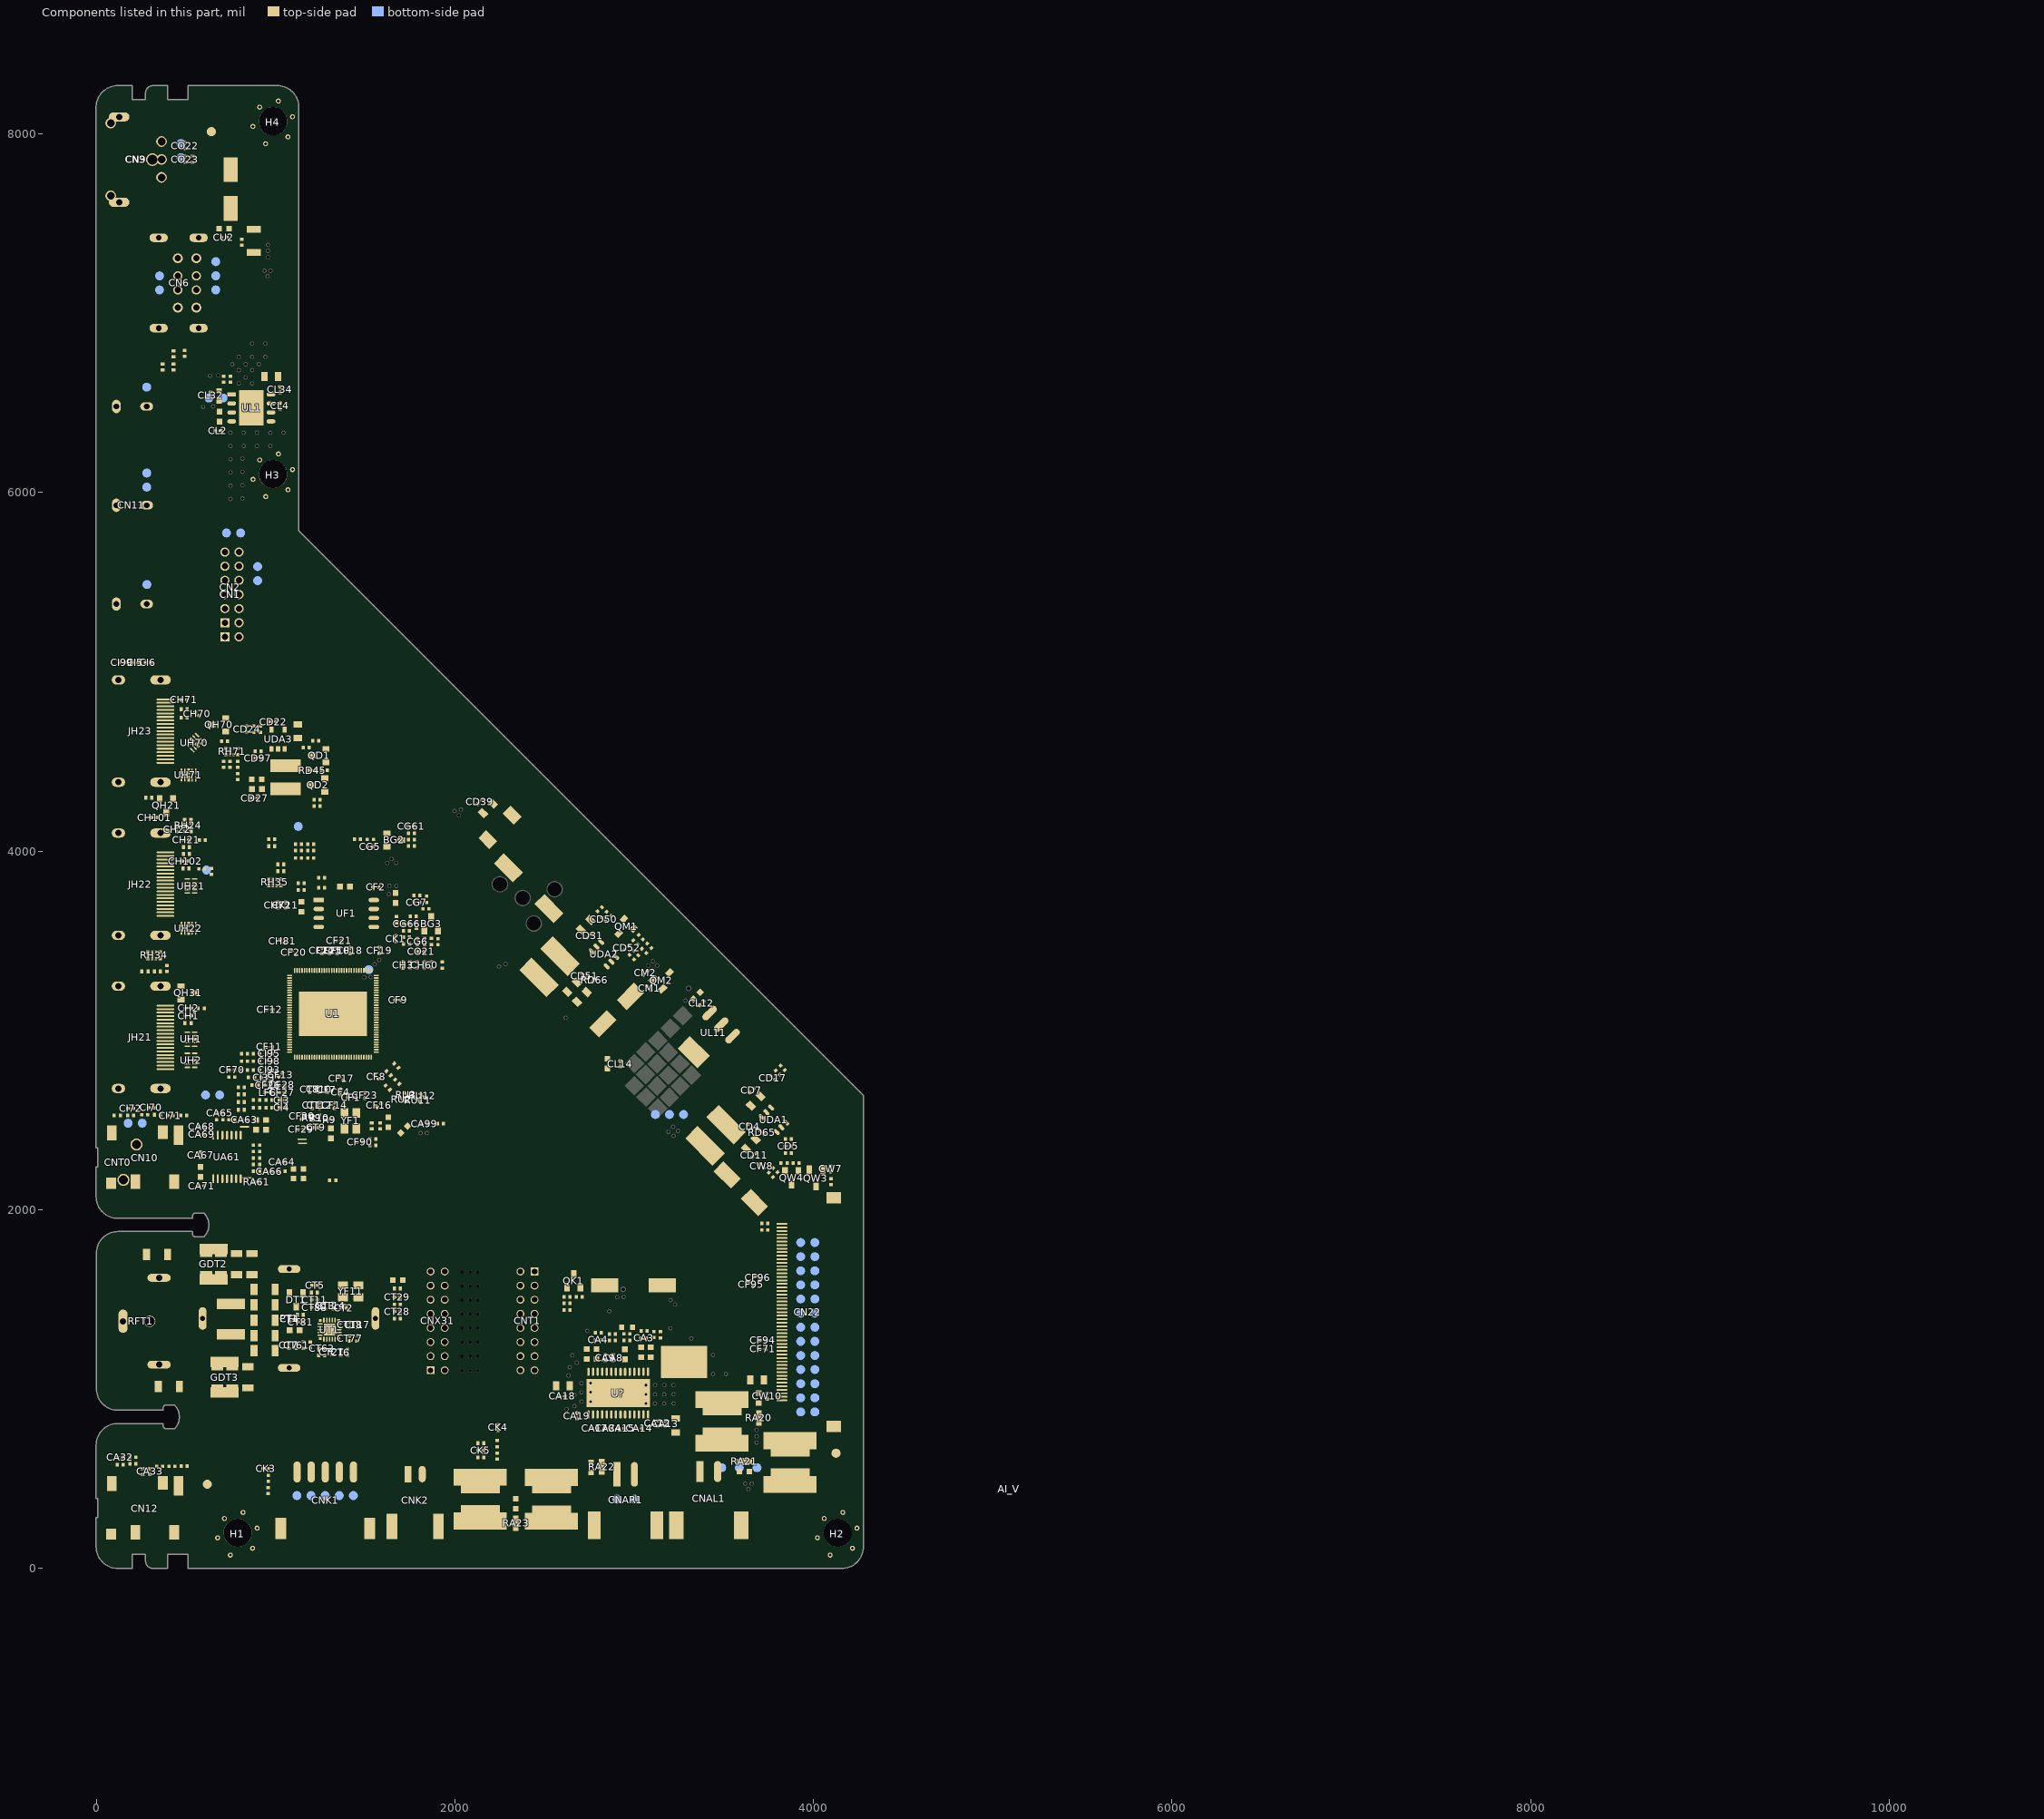
[diagram p0: the components of this part, seen from the top]
# Altium PCB MISC105950.PcbDoc (part 15 of 15)
Units mil, origin at the board's own origin, x right, y up, seen from the top; angles counter-clockwise.
Board outline 4280.62 x 8272.76 mil, 2 copper layers (TopLayer, BottomLayer), stack 61.855 mil thick; 541 components, 268 nets, 2324 pads, 1157 vias.

## Silkscreen, mask and mechanical layers (free items; w line width, h text height)
TopOverlay:
  drawing of 398 lines, arcs and shapes, not listed
  text "Solder Mask:" at 7538.71,8371.14 h60
  text "IPC SM-840" at 7951.21,8370.14 h60
  text "Silkscreen Color:" at 8717.21,8370.14 h60
  text "White" at 9196.21,8370.14 h60
  text "Units:" at 8717.21,8271.14 h60
  text "PTH Copper Thickness:" at 7538.71,8270.14 h60
  text "mm" at 8915.21,8269.64 h60
  text ">20um" at 8212.21,8269.14 h60
  text "4.2 --- 4.6" at 8717.87,8171.67 h60
  text "Dielectric Constant Er@1GHz To 1MHz:" at 7538.37,8171.17 h60
  text "Panel Size:" at 7532,8075.5 h60
  text "2L,2,63.26×214.50mm,FR4(TG130-CTI175),1OZ,Green,OSP,1.6mm" at 8184.37,8062.17 h60
  text "XXXXXXXXXX:" at 7830,8061.5 h60
  text "2L,2,51.80×25.20mm,FR4(TG130-CTI175),1OZ,Green,OSP,1.6mm" at 8184.87,7981.67 h60
  text "XX.XXXX:" at 7858,7975.5 h60
  text "Silkscreen on PTH:" at 7537.21,7871.14 h60
  text "Primary Side Retained;" at 8055.21,7870.14 h60
  text "Secondary Side  Removed for Soldering" at 8717.21,7868.64 h60
  text "Special Requirements" at 7536.19,7780.46 h60
  text "If engineering questions are not answered within 2 hours, call: PHONE_A" at 9422.87,7773.17 h60
  text "1. Lead-free hot air leveling (HAL_LF, Lead Free Hot Air Leveling)" at 8127.09,7676.87 h60
  text "2. Organic solderability preservative (OSP, Organic Solderability Preservatives)" at 8127.09,7592.87 h60
  text "3. Electroless nickel/immersion gold (ENIG, Electroless Nickel/Immersion Gold)" at 8125.59,7501.37 h60
  text "Plated Technics" at 7611.21,7466.64 h60
  text "4. Electroless nickel/immersion gold + gold finger (ENIG_G/F, Electroless Nickel/Immersion Gold + Gold Finger)" at 8127.09,7420.87 h60
  text "5. Gold plated (Gold_plated, Gold-plated)" at 8128.09,7340.37 h60
  text "6. Gold plated + gold finger (Gold_Plated_G/F, Gold-plated + Gold Finger)" at 8128.59,7262.37 h60
  text "Impedance Control" at 7540.94,7033.78 h60
  text "Target Impedance" at 8337.77,7033.88 h60
  text "Width & Clearance" at 9083.6,7033.65 h60
  text "Layer(s)" at 9851.91,7033.96 h60
  text "75 +/- 10% Ohm" at 8350.47,6927.68 h60
  text "G/12/15.8/12/G mil" at 9031.52,6927 h60
  text "layer 1" at 9842.41,6927.12 h60
  text "Single End Impedance" at 7540.94,6886.96 h60
  text "[ Zo ]" at 7764.44,6749.71 h60
  text "G/5/7/5/7/5/G mil" at 9041.52,6536 h60
  text "100 +/- 10% Ohm" at 8337.47,6534.99 h60
  text "layer 1" at 9853.4,6533.21 h60
  text "Differential Impedance" at 7540.8,6485.38 h60
  text "[ Zo ]" at 7763.93,6362.05 h60
  text "( G: Ground )" at 7674.01,6254.55 h60
  text "90 +/- 10% Ohm" at 8363.52,6237 h60
  text "layer 1&2" at 9849.4,6236.21 h60
  text "G/5/11/5/11/5/G mil" at 9041.52,6233.5 h60
  text "Common Mode Impedance" at 7520.58,6032.87 h60
  text "[ Zc ]" at 7768.58,5951.87 h60
  text "MAIN POWER" at 705,5810 h60
  text "INVERTER" at 745,5765 h60
  text "Refer to Gerber documents GTP&GBP for Stencil aperture design" at 8435.63,5687.68 h60
  text "Stencil" at 7534.87,5590.67 h60
  text "New (CN10, CNT0 compatible; note when opening the stencil)" at 8433.53,5493.12 h60
  text "Testing jig" at 7532.96,5395.02 h60
  text "New" at 8435.63,5385.92 h60
  text "Wave-soldering jig" at 7535.17,5296.78 h60
  text "New (when CNX31, CNT1 pass wave soldering, a wave-soldering fixture is required)" at 8425,5297 h60
  text "Solder paste" at 8433.15,5195 h60
  text "Production process" at 7533.65,5193.5 h60
  text "[Process and notes]" at 7713.87,5108.67 h60
  text "SMD parts 3.5mm from PCB edge; production must control specially" at 8432.87,5109.17 h60
  text "Special requirements" at 7534.65,4995.5 h60
  text "SMD parts higher than 2mm on the wave-soldering side" at 7534.37,4894.17 h60
  text "Package attention" at 7534.03,4797.95 h60
  text "[Easily damaged parts]" at 7775.37,4713.17 h60
  text "New footprint matching" at 7534.03,4597.95 h60
  text "RFT1, PT1 are temporary footprints" at 8431.52,4543 h60
  text "[New component footprint]" at 7761.37,4514.17 h60
  text "(Automated Testing Support)" at 7852.37,4399.67 h45
  text "Automated test support" at 7533.87,4396.17 h60
  text "Yes" at 8432.37,4340.17 h60
  text "[Reserved suction cup and press bar positions]" at 7694.37,4311.67 h60
  text "Layer Stack Up Detail for" at 7674.97,3952.14 h100
  text ".Pcb_File_Name_No_Path" at 8735.79,3952.14 h100
  text "Layer" at 7839.33,3804.41 h50
  text "Gerber" at 8211.04,3804.41 h50
  text "Layer" at 8522.19,3804.41 h50
  text "Layer" at 9158.43,3804.41 h50
  text "Copper" at 9947.33,3804.41 h50
  text "Dielectric" at 10259.11,3804.41 h50
  text "Stack up" at 9158.43,3753.53 h50
  text "Height" at 10259.11,3753.53 h50
  text "Name" at 7839.33,3752.03 h50
  text "Document" at 8211.04,3752.03 h50
  text "Ordor" at 8522.19,3752.03 h50
  text "Thickness" at 9947.33,3752.03 h50
  text "TopOverlay" at 7839.03,3519.18 h60
  text ".GTO" at 8248.6,3516.62 h60
  text "0.4mil" at 10256.43,3431.59 h60
  text "1" at 8575.39,3328.44 h60
  text "1.4mil" at 9960.39,3328.38 h60
  text "2" at 8575.45,3115.4 h60
  text "1.4mil" at 9958.68,3114.39 h60
  text "0.4mil" at 10259.1,3019.71 h60
  text "LVDS" at 4195.3,2126.1 h60 r90
  text "ALL SMT" at 1966.7,45.6 h180
  text "SPEAKER _L" at 3275.6,45.2 h60
  text "SPEAKER _R" at 2788.3,39.2 h60
  text "IR&KEY" at 1185.1,35 h60
  text "KEY" at 1724.1,29.1 h60
BottomOverlay:
  drawing of 184 lines, arcs and shapes, not listed
  text "COAX OUT/OPTICAL OUT" at 200.6,7422 h60 r270
  text "USB IN" at 101.9,7093.1 h60 r270
  text "AV IN/YPBPR AUDIO IN" at 162.2,5936.8 h60 r270
  text "BL_ON" at 652.8,5655.1 h50
  text "ADJ/PWM" at 488.3,5652.9 h50
  text "PW_ON" at 656.91,5570.73 h50
  text "GND" at 474.91,5568.43 h50
  text "NC" at 470.9,5493.5 h50
  text "ADIM" at 641.9,5492.9 h50
  text "GND" at 503,5414.9 h50
  text "GND" at 659,5415.4 h50
  text "12V/15V" at 671.5,5338.2 h50
  text "GND" at 487.9,5337.3 h50
  text "12V/15V" at 485.3,5255 h50
  text "12V/15V" at 670.1,5252.4 h50
  text "12V/15V" at 630.4,5172.8 h50
  text "GND" at 448.4,5170.5 h50
  text "HDMI3 IN" at 36.6,4524.9 h60 r270
  text "HDMI2 IN" at 35,3742.6 h60 r270
  text "S.P" at 25.8,3567.3 h90 r270
  text ".GBO" at 8249.22,2924.1 h60
  text "BottomOverlay" at 7827.55,2923.11 h60
  text "HDMI1(ARC) IN" at 38.1,2781.7 h60 r270
  text "YPBPR IN" at 536.21,2178.28 h60
  text "RF IN" at 39.48,1316.39 h60 r270
  text "LOUT-" at 3385.9,631.3 h50 r270
  text "LOUT+" at 3322.7,625 h50 r270
  text "ROUT-" at 2985.66,599.28 h50 r270
  text "ROUT+" at 2890.7,588.7 h50 r270
  text "GND" at 1881,545 h50
  text "KEY" at 1764.7,542 h50
  text "IR" at 1164.6,229.7 h50 r270
  text "3.3V" at 1114.5,215 h50 r270
  text "LED" at 1261.1,214.3 h50 r270
  text "KEY" at 1309,214.3 h50 r270
  text "GND" at 1209.5,209.9 h50 r270
  text "EARPHONE OUT" at 453.4,182.9 h60
  text "LINE OUT" at 366.7,102.7 h60
TopPaste:
  rectangle: 7673.59,3594.48 7803.79,3673.22
  rectangle: 198.7,7809.2 281.5,7907.3
  region: 171,2253.56 123,2253.56 108.5,2239.06 108.5,2211.56 132,2188.06 159.06,2188.06 185,2214 185,2239.56
  lines w5: 8224.49,3594.48 8224.49,3673.22 ; 7673.59,3594.48 7673.59,3673.22 8405.62,3673.22 8405.62,3594.48 7673.59,3594.48
  text "TopPaste" at 7839.03,3615.71 h60
  text ".GTP" at 8248.6,3613.58 h60
BottomPaste:
  rectangle: 7673.59,2806.92 7803.79,2885.66
  lines w5: 8224.49,2806.92 8224.49,2885.66 ; 7673.59,2806.92 7673.59,2885.66 8405.62,2885.66 8405.62,2806.92 7673.59,2806.92
  text "BottomPaste" at 7826.39,2829.9 h60
  text ".GBP" at 8249.49,2824.78 h60
TopSolder:
  rectangle: 7673.59,3404.53 7803.79,3483.27
  lines w5: 8224.49,3404.53 8224.49,3483.27 ; 7673.59,3404.53 7673.59,3483.27 8405.62,3483.27 8405.62,3404.53 7673.59,3404.53
  text "TopSolder" at 7839.53,3424.63 h60
  text ".GTS" at 8248.6,3422.98 h60
BottomSolder:
  rectangle: 7673.59,2994.72 7803.79,3073.46
  region: 1968.4,1049.81 1968.4,971.47 1939.32,923 1859.68,923 1830.6,971.47 1830.6,1049.81
  region: 2469.66,1049.75 2469.66,971.41 2422.41,892.67 2379.11,892.67 2331.86,971.41 2331.86,1049.75
  lines w5: 8224.49,2994.72 8224.49,3073.46 ; 7673.59,2994.72 7673.59,3073.46 8405.62,3073.46 8405.62,2994.72 7673.59,2994.72
  lines w27.56: 210.15,2938.08 338.78,3066.7 ; 210.15,3021.59 255.26,3066.7 ; 210.15,3792.41 338.78,3921.03 ; 210.15,3875.92 255.26,3921.03 ; 210.15,4646.74 338.78,4775.36 ; 210.15,4730.25 255.26,4775.36 ; 210.22,2854.63 421.97,3066.38 ; 210.22,3708.96 421.97,3920.71 ; 210.22,4563.29 421.97,4775.04 ; 293.81,2854.7 422.65,2983.54 ; 293.81,3709.03 422.65,3837.87 ; 293.81,4563.36 422.65,4692.2 ; 377.33,2854.7 422.65,2900.03 ; 377.33,3709.03 422.65,3754.36 ; 377.33,4563.36 422.65,4608.69
  text "BottomSolder" at 7826.39,3016.31 h60
  text ".GBS" at 8248.57,3015.42 h60
3D和装配:
  lines w5: 50.61,2695.01 582.1,2695.01 582.1,3226.51 50.61,3226.51 50.61,2695.01 ; 50.61,3549.34 582.1,3549.34 582.1,4080.84 50.61,4080.84 50.61,3549.34 ; 50.61,4403.67 582.1,4403.67 582.1,4935.17 50.61,4935.17 50.61,4403.67
  text "2L,2,63.26×214.50mm,FR4(TG130-CTI175),1OZ,Green,OSP,1.6mm,4,64,81.3%,1624,0.4mm" at 8184.37,8062.17 h60
  text "2L,2,51.80×25.20mm,FR4(TG130-CTI175),1OZ,Green,OSP,1.6mm,4,64,81.3%,1624,0.4mm" at 8184.87,7981.67 h60
自动测试:
  circle w6: c3435.52,1472.17 r196.85
  circle w6: c595.02,6014.17 r196.85
  circle w6: c596.15,6014.17 r236.22
  circle w6: c1555.85,4758.34 r196.85
  circle w6: c1556.98,4758.34 r236.22
  circle w6: c778.52,3386.67 r196.85
  circle w6: c779.65,3386.67 r236.22
  circle w6: c2342.52,2795.67 r196.85
  circle w6: c2343.65,2795.67 r236.22
  circle w6: c3073.65,2057.17 r236.22
  circle w6: c3072.52,2057.17 r196.85
  circle w6: c899.15,7040 r196.85
顶层限制:
  drawing of 4128 lines, arcs and shapes, not listed
  text "28.6" at 562.99,8601.63 h98.43
  text "25" at 492.13,8365.41 h98.43
  text "1.5" at -505.8,7497.38 h98.43
  text "25" at 411.2,6220.76 h98.43
  text "1.5" at -509.8,4972.38 h98.43
  text "210" at -3064.65,4084.65 h98.43
  text "205" at -2828.43,3986.22 h98.43
  text "199.6" at -2592.21,3879.92 h98.43
  text "182.1" at -2355.99,3535.43 h98.43
  text "155" at -2119.77,3001.97 h98.43
  text "150.6" at -1883.55,2915.36 h98.43
  text "137.96" at 4684.7,2675.76 h98.43
  text "1.5" at -365.49,2542.9 h98.43
  text "2.25" at -4350.24,2464.06 h98.43
  text "5" at -4226.22,2414.15 h98.43 r225
  text "阴忧蛭饪墙鹗舨糠?" at 118.11,2396.65 h23.62 r270
  text "118.6" at -1647.33,2285.43 h98.43
  text "4.45" at -4308.89,2140.75 h98.43
  text "96.9" at -1411.11,1858.27 h98.43
  text "75.2" at -1273.96,1431.1 h98.43
  text "9.3" at -3946.98,1378.53 h98.43 r270
  text "58.2" at -1155.85,1096.46 h98.43
  text "57.5" at -938.67,1082.68 h98.43
  text "11.53" at -225.79,955.68 h98.43
  text "6.3" at -4775.37,934.26 h98.43
  text "36.25" at 4480.52,664.46 h98.43
  text "35.01" at -702.45,639.95 h98.43
  text "2.25" at -4350.24,507.36 h98.43
  text "5" at -4226.22,457.46 h98.43 r225
  text "阴忧蛭饪墙鹗舨糠?" at 118.11,439.96 h23.62 r270
  text "8.5" at -690.64,383.86 h98.43
  text "4.45" at -4308.89,184.06 h98.43
  text "IR&KEY" at 1140.62,53.2 h50
  text "KEY" at 1700.14,53.2 h50
  text "5" at -230.01,49.21 h98.43
  text "20" at 300.7,-196.12 h98.43
  text "1.6" at -4182.58,-197.49 h98.43
  text "4.38" at 1037.7,-242.62 h98.43
  text "105" at 2066.93,-434.6 h98.43
  text "106.5" at 2096.42,-670.82 h98.43
  text "108.6" at 2151.07,-874.93 h98.43
底层限制:
  drawing of 380 lines, arcs and shapes, not listed
  text "25" at 413.28,5615.88 h98.43
附加说明:
  lines w5: -190,8051.04 1356.5,8051.04 ; -95.16,216.54 4617.5,216.54 ; 10817.53,7894.99 11947.53,7894.99 ; 10817.53,8002.32 11947.53,8002.32 ; 10817.53,8109.65 11947.53,8109.65 ; 10817.53,8216.99 11947.53,8216.99 ; 10817.53,8324.32 12248.03,8324.32 ; 11118.03,7787.65 11118.03,8431.65 ; 11947.53,7787.65 11947.53,8431.65 ; 12301.03,7894.99 14269.53,7894.99 ; 12301.03,8002.32 14269.53,8002.32 ; 12301.03,8109.65 14269.53,8109.65 ; 12301.03,8216.99 14269.53,8216.99 ; 12301.03,8324.32 14269.53,8324.32 ; 12405.53,7787.65 12405.53,8324.32 ; 10817.53,7787.65 10817.53,8431.65 12248.03,8431.65 12248.03,7787.65 10817.53,7787.65 ; 12301.03,7787.65 14269.53,7787.65 14269.53,8431.65 12301.03,8431.65 12301.03,7787.65
  text "Keep the description brief, so derived projects or board revisions can inherit it:" at 12705.37,8386.67 h35
  text "Template date:" at 9550.37,8369.67 h60
  text "2019.08.22" at 9872.37,8366.17 h60
  text "Version cycle number" at 10839.37,8358.5 h60
  text "PCB designer" at 11394.87,8358 h60
  text "Customer" at 12057.87,8358.5 h60
  text "Special remarks" at 12332.37,8358.5 h60
  text "e.g. new or special design rules: hole spacing for Bangladesh region; special safety distances; special stack-up not allowed to change; support chain; designated factory..." at 12704.87,8341.17 h35
  text "Board utilization:" at 9549.87,8272.67 h60
  text "8X%" at 9872.37,8268.67 h60
  text "(To be filled in for non-TV division projects)" at 10062.37,8268.67 h60
  text "XXXXXX." at 10858.87,8251.5 h60
  text "CK&HMZ" at 11162.87,8250.67 h60
  text "1" at 12342.37,8251.5 h60
  text "2" at 12342.32,8144.34 h60
  text "COMPANY_A" at 11986.87,8041.17 h60
  text "3" at 12342.37,8037.34 h60
  text "4" at 12342.37,7929.34 h60
  text "5" at 12342.37,7822.34 h60
  text "① Panel production, ship single boards" at 8984.37,7804.67 h30
  text "Special board requirements; leave blank if none;" at 8140.53,7772.01 h60
  text "Reference:" at 8849.37,7771.17 h60
  text "② 4-up panel production, ship 2-up panels" at 8983.87,7760.67 h30
  text "The remark items below must be copied to the TopOverlay layer; one or two remark items" at 9137.87,5191.17 h60
  text "Only one barcode position on board; the other barcode to be attached to a component" at 10656.5,5188.27 h60
  text "No barcode position on board; barcode to be attached to a component" at 10656.5,5109.07 h60
  text "Customer special requirements; special process requirements; leave blank if none" at 8430.92,4996.21 h60
  text "Height value and designators of parts over 2mm on the solder side; leave blank if none" at 8430.92,4896.21 h60
  text "Designators of easily damaged parts; leave blank if none" at 8429.15,4750.05 h60
  text "X.XXXX.XXX Stencil Revision Explanation" at 7508.12,2429.08 h60
  text "X.XXXX.XXX Testing jig Revision Explanation" at 7507.62,2360.08 h60
  text "X.XXXX.XXX Wave-soldering jig Revision Explanation" at 7507.12,2292.08 h60
DrillDrawing:
  text ".Legend" at 7513.19,8489.89 h60